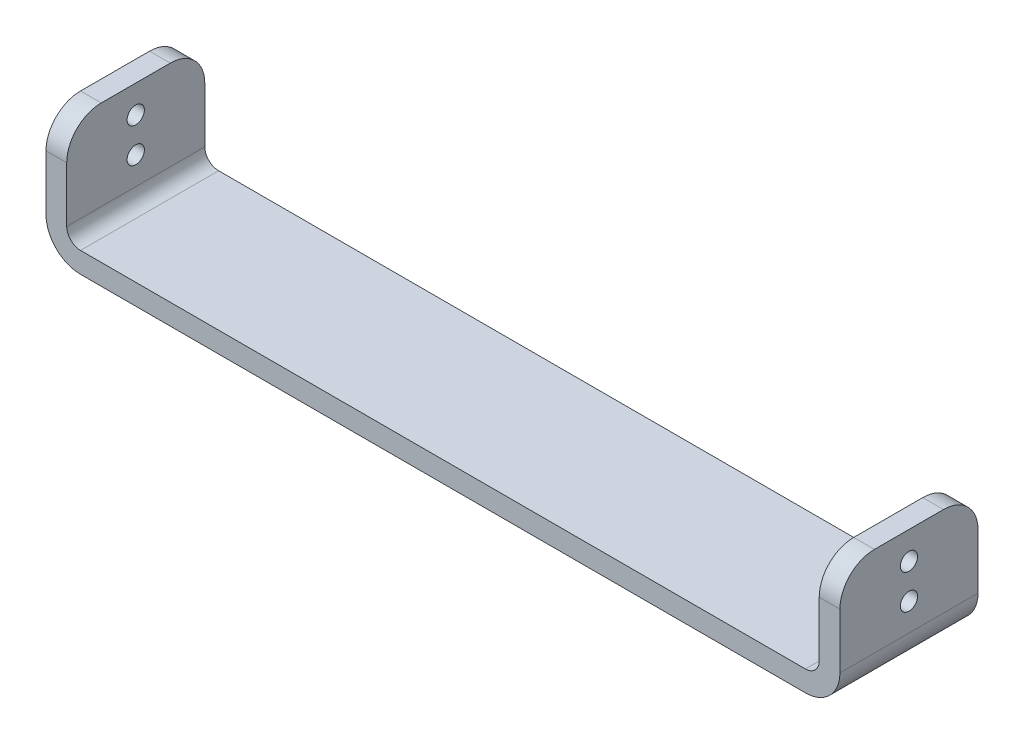
SolidWorks part; units mm, degrees
ref_plane "Front Plane" through (0, 0, 0) normal (0, 0, 1) x (1, 0, 0)
ref_plane "Top Plane" through (0, 0, 0) normal (0, 1, 0) x (1, 0, 0)
ref_plane "Right Plane" through (0, 0, 0) normal (1, 0, 0) x (0, 0, -1)
sketch "Sketch1" plane through (0, 0, 0) normal (0, 1, 0) x (1, 0, 0)
  line L5 (-57.5, -10) -> (57.5, -10)
  line L6 (-57.5, -10) -> (-57.5, 10)
  line L7 (-57.5, 10) -> (57.5, 10)
  line L8 (57.5, -10) -> (57.5, 10)
  line L9 (-57.5, -10) -> (57.5, 10) construction
  line L10 (-57.5, 10) -> (57.5, -10) construction
  point P0 (0, 0)
  dimension "D1" = 115
  dimension "D2" = 20
extrude "Boss-Extrude1" add sketch "Sketch1" along normal blind 3
sketch "Sketch2" plane through (0, 3, 0) normal (0, 1, 0) x (1, 0, 0)
  line L0 (-57.5, -10) -> (57.5, -10) construction
  line L1 (-57.5, 10) -> (-54.5, 10)
  line L2 (-57.5, 10) -> (-57.5, -10)
  line L3 (-57.5, -10) -> (-54.5, -10)
  line L4 (-54.5, 10) -> (-54.5, -10)
  line L6 (57.5, 10) -> (54.5, 10)
  line L7 (57.5, 10) -> (57.5, -10)
  line L8 (57.5, -10) -> (54.5, -10)
  line L9 (54.5, 10) -> (54.5, -10)
  dimension "D1" = 3
  dimension "D2" = 3
extrude "Boss-Extrude2" add sketch "Sketch2" along normal blind 15
fillet "Fillet1" radius 2 2 edges at (54.5, 3, 0) (-54.5, 3, 0)
fillet "Fillet2" radius 5 2 edges at (57.5, 0, 0) (-57.5, 0, 0)
hole_wizard "M3 Tapped Hole1" positions "Sketch3" profile "Sketch4" tap size "M3" standard "GB" end condition through all
sketch "Sketch3" plane through (-57.5, 0, 0) normal (-1, 0, 0) x (0, 0, 1)
  line L1 (-10, 18) -> (10, 18) construction
  point P0 (0, 14)
  point P11 (0, 9)
  dimension "D1" = 4
  dimension "D2" = 5
sketch "Sketch4" plane through (-57.5, 14, 0) normal (0, 1, 0) x (0, 0, 1)
  line L0 (0, 0) -> (0, 115)
  line L1 (0, 115) -> (1.25, 115)
  line L2 (1.25, 115) -> (1.25, 0)
  line L5 (1.25, 0) -> (0, 0)
  line L11 (0, -6.35) -> (0, 107.95) construction
  dimension "通孔螺纹孔钻头直径" = 2.5
  dimension "通孔螺纹孔钻头深度" = 115
cosmetic thread "Tapped hole thread 1"
cosmetic thread "Tapped hole thread 2"
fillet "Fillet3" radius 5 4 edges at (-56, 18, 10) (-56, 18, -10) (56, 18, 10) (56, 18, -10)
